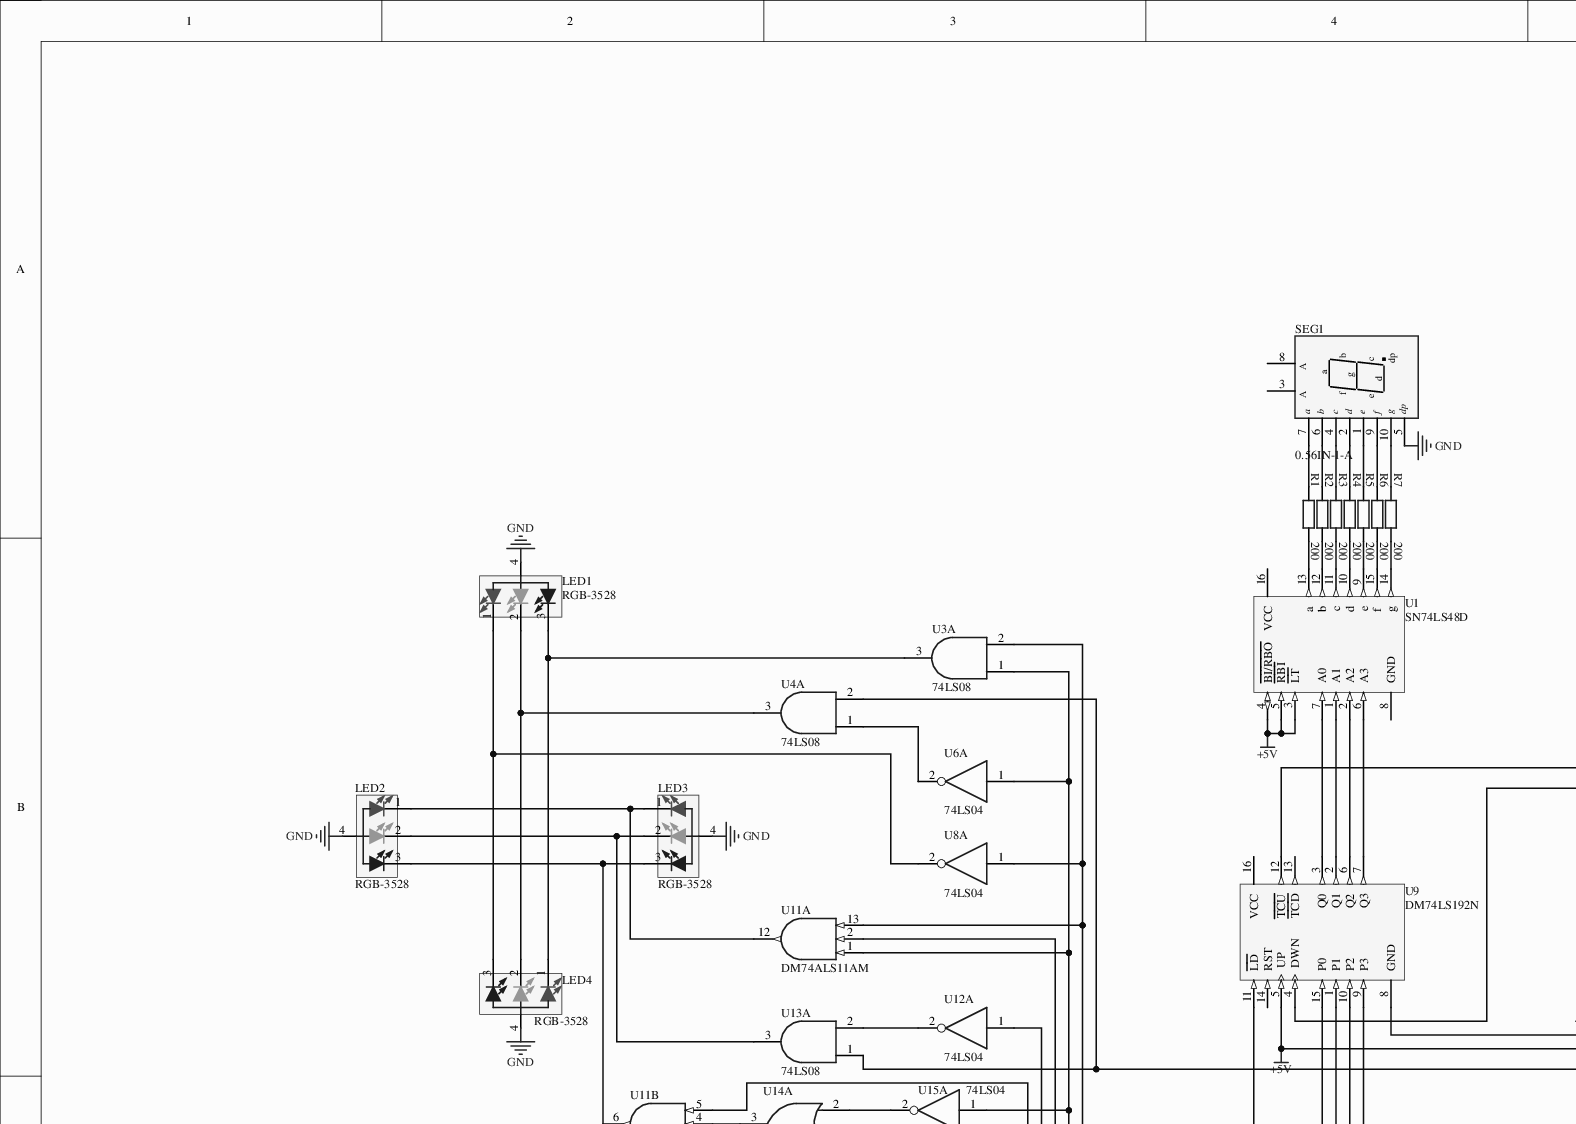
[diagram p0: MISC82158-6.SchDoc, top left]
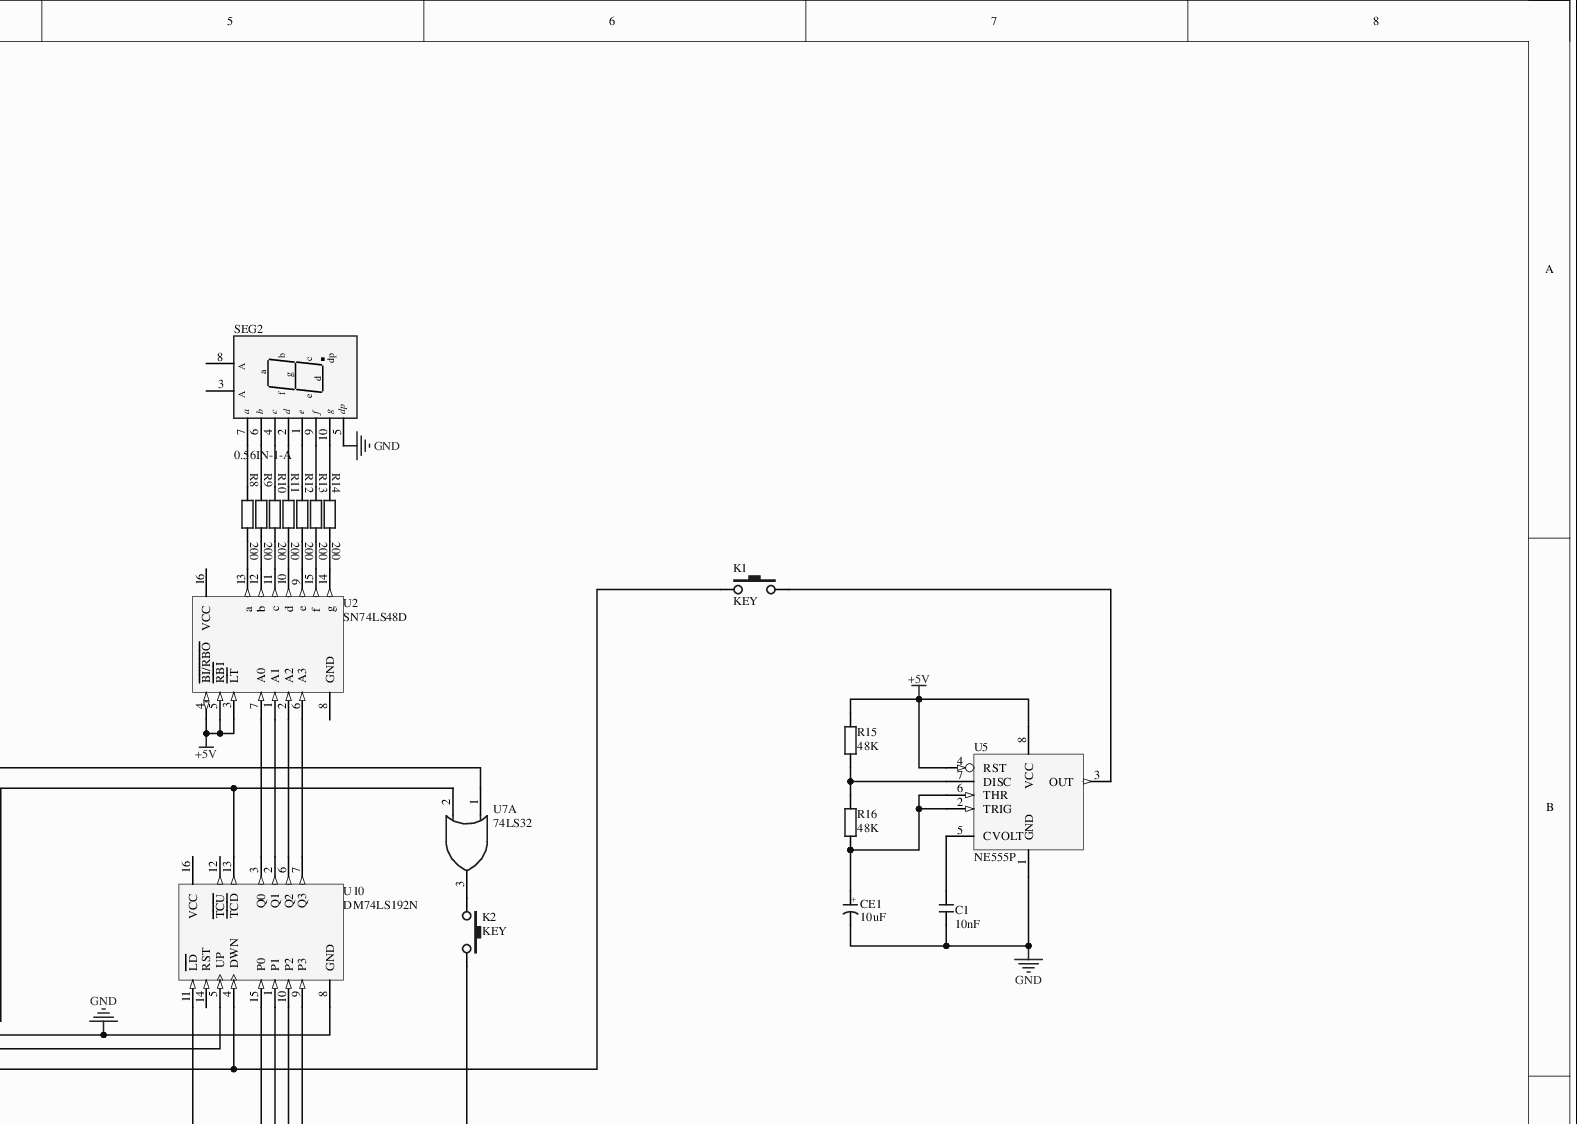
[diagram p1: MISC82158-6.SchDoc, top right]
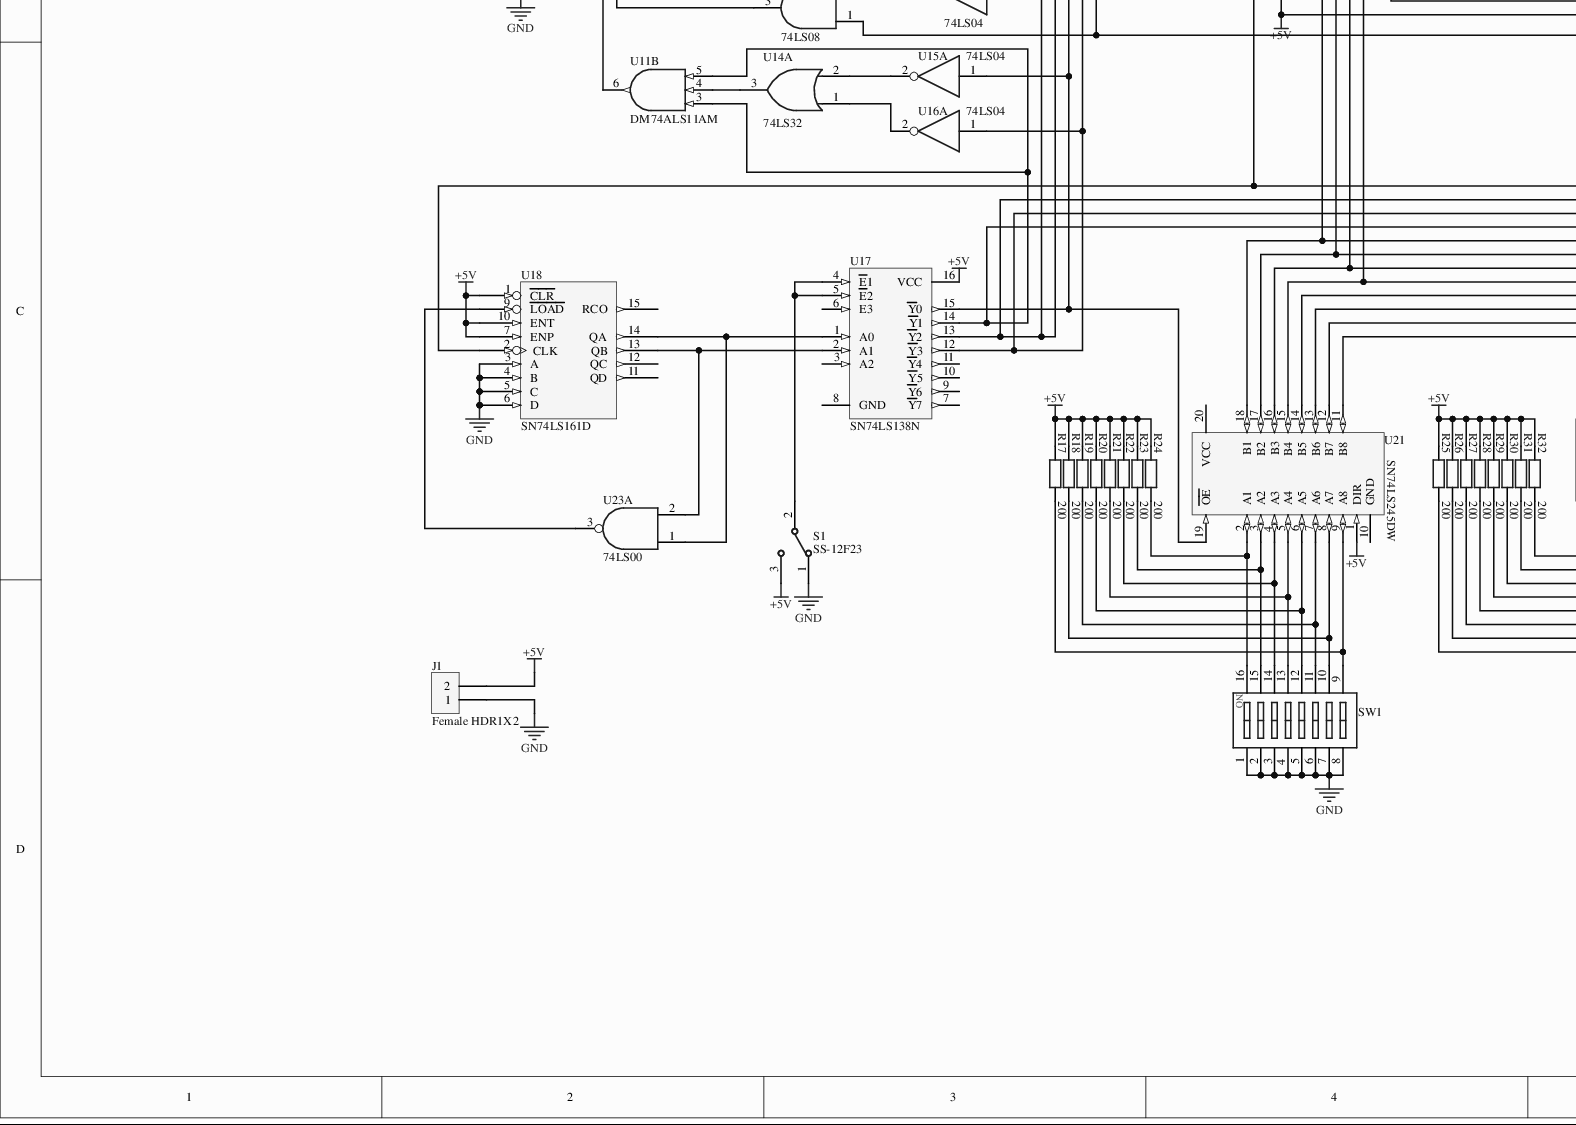
[diagram p2: MISC82158-6.SchDoc, bottom left]
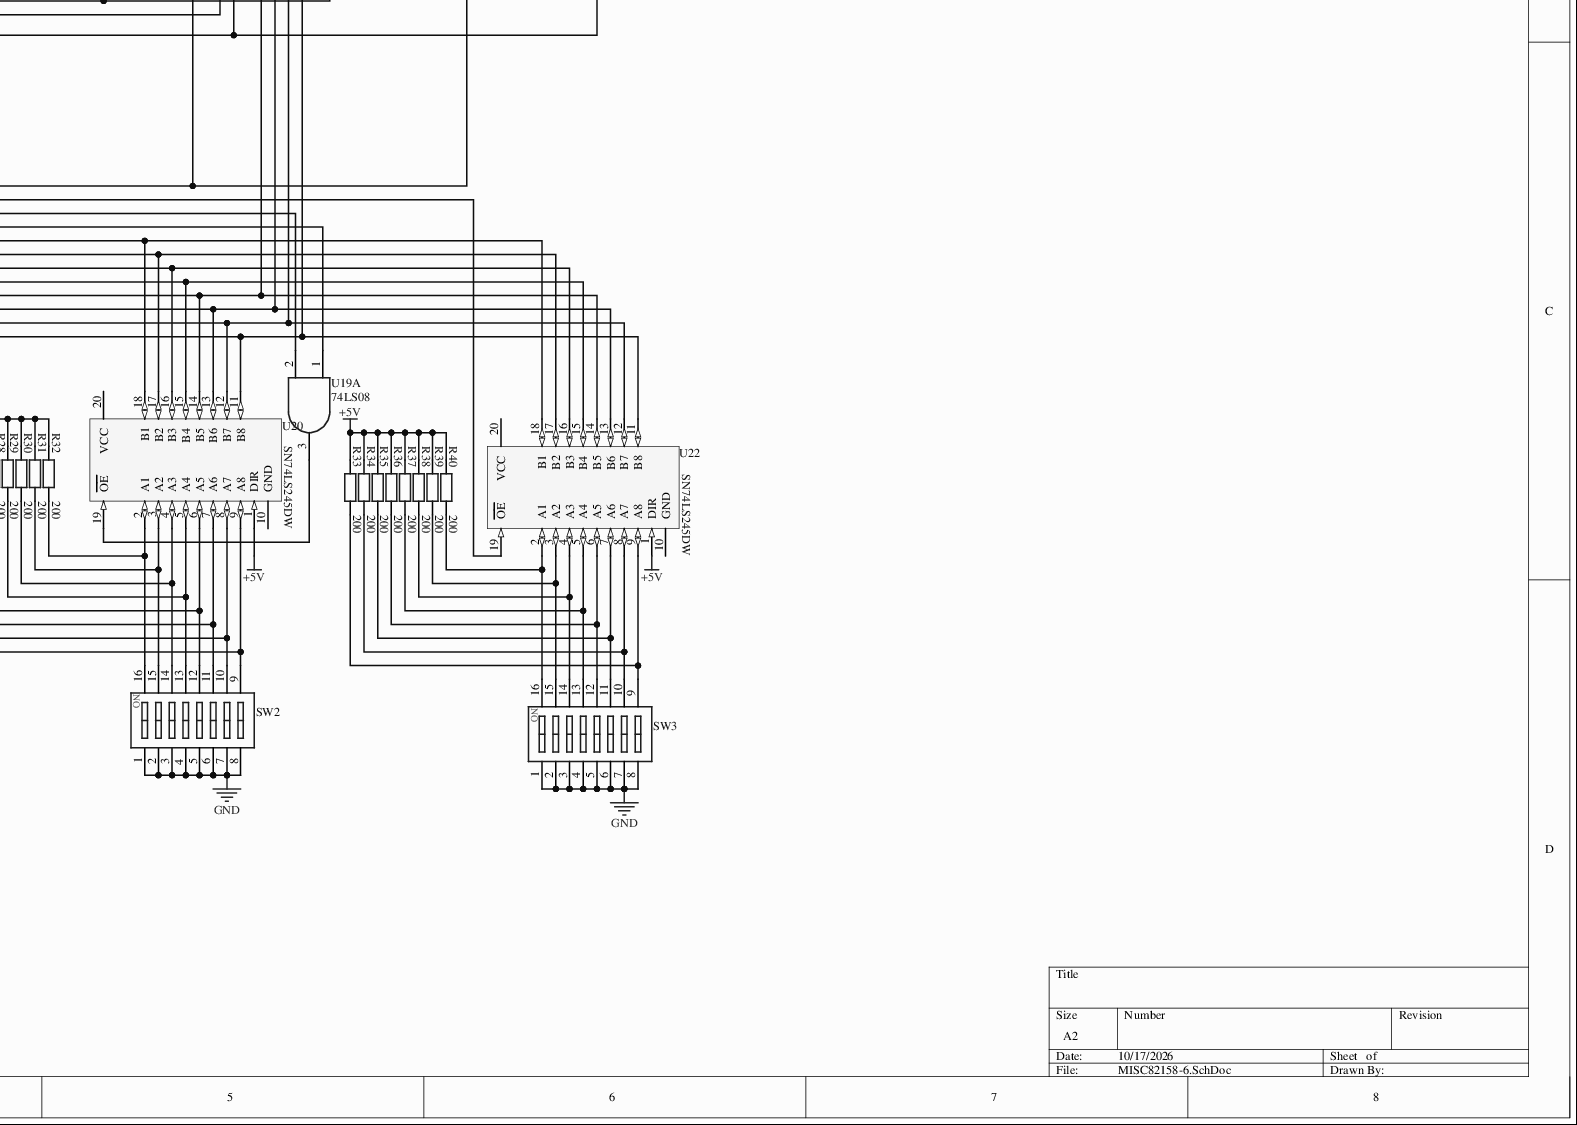
[diagram p3: MISC82158-6.SchDoc, bottom right]
# Altium project MISC82158-9.PrjPcb
1 sheet, 78 parts. Net scope: global (net labels, ports and power ports of the same name join across sheets).
Board file: MISC82158.PcbDoc

## Sheet MISC82158-6.SchDoc
size A2

### Parts
C1  10nF  [CC 1.8*3.6]
CE1  10uF  [CAP 1.5*4*8]
J1  Female HDR1X2  [Fe-HDR1X2/2.54-S]
K1  KEY  [DIP-3X6X4.3]
K2  KEY  [DIP-3X6X4.3]
LED1  RGB-3528  [Fe-HDR1X4/2.54-S]
LED2  RGB-3528  [Fe-HDR1X4/2.54-S]
LED3  RGB-3528  [Fe-HDR1X4/2.54-S]
LED4  RGB-3528  [Fe-HDR1X4/2.54-S]
R1  200  [RS 1/4W]
R2  200  [RS 1/4W]
R3  200  [RS 1/4W]
R4  200  [RS 1/4W]
R5  200  [RS 1/4W]
R6  200  [RS 1/4W]
R7  200  [RS 1/4W]
R8  200  [RS 1/4W]
R9  200  [RS 1/4W]
R10  200  [RS 1/4W]
R11  200  [RS 1/4W]
R12  200  [RS 1/4W]
R13  200  [RS 1/4W]
R14  200  [RS 1/4W]
R15  48K  [RS 1/4W]
R16  48K  [RS 1/4W]
R17  200  [RS 1/4W]
R18  200  [RS 1/4W]
R19  200  [RS 1/4W]
R20  200  [RS 1/4W]
R21  200  [RS 1/4W]
R22  200  [RS 1/4W]
R23  200  [RS 1/4W]
R24  200  [RS 1/4W]
R25  200  [RS 1/4W]
R26  200  [RS 1/4W]
R27  200  [RS 1/4W]
R28  200  [RS 1/4W]
R29  200  [RS 1/4W]
R30  200  [RS 1/4W]
R31  200  [RS 1/4W]
R32  200  [RS 1/4W]
R33  200  [RS 1/4W]
R34  200  [RS 1/4W]
R35  200  [RS 1/4W]
R36  200  [RS 1/4W]
R37  200  [RS 1/4W]
R38  200  [RS 1/4W]
R39  200  [RS 1/4W]
R40  200  [RS 1/4W]
S1  SS-12F23  [MSK-12C01-07]
SEG1  0.56IN-1-A  [0.56IN-1P]
SEG2  0.56IN-1-A  [0.56IN-1P]
SW1  SW-8P  [CSW DIP-8P]  (value not drawn)
SW2  SW-8P  [CSW DIP-8P]  (value not drawn)
SW3  SW-8P  [CSW DIP-8P]  (value not drawn)
U1  SN74LS48D  [SOP16]
U2  SN74LS48D  [SOP16]
U3  74LS08  [DIP14]  (part A of 4)
U4  74LS08  [DIP14]  (part A of 4)
U5  NE555P  [DIP8]
U6  74LS04  [DIP14]  (part A of 6)
U7  74LS32  [DIP14]  (part A of 4)
U8  74LS04  [DIP14]  (part A of 6)
U9  DM74LS192N  [DIP16]
U10  DM74LS192N  [DIP16]
U11  DM74ALS11AM  [DIP16]  (parts A,B of 3)
U12  74LS04  [DIP14]  (part A of 6)
U13  74LS08  [DIP14]  (part A of 4)
U14  74LS32  [DIP14]  (part A of 4)
U15  74LS04  [DIP14]  (part A of 6)
U16  74LS04  [DIP14]  (part A of 6)
U17  SN74LS138N  [DIP16]
U18  SN74LS161D  [DIP16]
U19  74LS08  [DIP14]  (part A of 4)
U20  SN74LS245DW  [SOP20]
U21  SN74LS245DW  [SOP20]
U22  SN74LS245DW  [SOP20]
U23  74LS00  [DIP14]  (part A of 4)

### Nets
+5V: J1.2 R15.1 R17.2 R18.2 R19.2 R20.2 R21.2 R22.2 R23.2 R24.2 R25.2 R26.2 R27.2 R28.2 R29.2 R30.2 R31.2 R32.2 R33.2 R34.2 R35.2 R36.2 R37.2 R38.2 R39.2 R40.2 S1.3 U1.3(~{LT}) U1.4(~{BI/RBO}) U1.5(~{RBI}) U2.3(~{LT}) U2.4(~{BI/RBO}) U2.5(~{RBI}) U5.4(RST) U5.8(VCC) U9.5(UP) U10.5(UP) U17.16(VCC) U18.1(~{CLR}) U18.7(ENP) U18.10(ENT) U20.1(DIR) U21.1(DIR) U22.1(DIR)
GND: C1.1 CE1.2(K) J1.1 LED1.4(A) LED2.4(A) LED3.4(A) LED4.4(A) S1.1 SEG1.5 SEG2.5 SW1.1 SW1.2 SW1.3 SW1.4 SW1.5 SW1.6 SW1.7 SW1.8 SW2.1 SW2.2 SW2.3 SW2.4 SW2.5 SW2.6 SW2.7 SW2.8 SW3.1 SW3.2 SW3.3 SW3.4 SW3.5 SW3.6 SW3.7 SW3.8 U5.1(GND) U9.8(GND) U10.8(GND) U11.7(GND) U18.3(A) U18.4(B) U18.5(C) U18.6(D) U18.8(GND)
VCC: U11.14(VCC) U18.16(VCC)
NetC1_2: C1.2 U5.5(CVOLT)
NetCE1_1: CE1.1(A) R16.2 U5.2(TRIG) U5.6(THR)
NetK1_1: K1.1 U4.2(B) U10.4(DWN) U13.1(A)
NetK1_3: K1.3 U5.3(OUT)
NetK2_1: K2.1 U7.3(Y)
NetK2_3: K2.3 U9.11(~{LD}) U10.11(~{LD}) U18.2(CLK)
NetLED1_1: LED1.1(RED_K) LED4.3(BULE_K) U8.2(Y)
NetLED1_2: LED1.2(GREEN_K) LED4.2(GREEN_K) U4.3(Y)
NetLED1_3: LED1.3(BULE_K) LED4.1(RED_K) U3.3(Y)
NetLED2_1: LED2.1(RED_K) LED3.1(RED_K) U11.12(Y)
NetLED2_2: LED2.2(GREEN_K) LED3.2(GREEN_K) U13.3(Y)
NetLED2_3: LED2.3(BULE_K) LED3.3(BULE_K) U11.6(Y)
NetR1_1: R1.1 U1.13(a)
NetR1_2: R1.2 SEG1.7
NetR2_1: R2.1 U1.12(b)
NetR2_2: R2.2 SEG1.6
NetR3_1: R3.1 U1.11(c)
NetR3_2: R3.2 SEG1.4
NetR4_1: R4.1 U1.10(d)
NetR4_2: R4.2 SEG1.2
NetR5_1: R5.1 U1.9(e)
NetR5_2: R5.2 SEG1.1
NetR6_1: R6.1 U1.15(f)
NetR6_2: R6.2 SEG1.9
NetR7_1: R7.1 U1.14(g)
NetR7_2: R7.2 SEG1.10
NetR8_1: R8.1 U2.13(a)
NetR8_2: R8.2 SEG2.7
NetR9_1: R9.1 U2.12(b)
NetR9_2: R9.2 SEG2.6
NetR10_1: R10.1 U2.11(c)
NetR10_2: R10.2 SEG2.4
NetR11_1: R11.1 U2.10(d)
NetR11_2: R11.2 SEG2.2
NetR12_1: R12.1 U2.9(e)
NetR12_2: R12.2 SEG2.1
NetR13_1: R13.1 U2.15(f)
NetR13_2: R13.2 SEG2.9
NetR14_1: R14.1 U2.14(g)
NetR14_2: R14.2 SEG2.10
NetR15_2: R15.2 R16.1 U5.7(DISC)
NetR17_1: R17.1 SW1.9 U21.9(A8)
NetR18_1: R18.1 SW1.10 U21.8(A7)
NetR19_1: R19.1 SW1.11 U21.7(A6)
NetR20_1: R20.1 SW1.12 U21.6(A5)
NetR21_1: R21.1 SW1.13 U21.5(A4)
NetR22_1: R22.1 SW1.14 U21.4(A3)
NetR23_1: R23.1 SW1.15 U21.3(A2)
NetR24_1: R24.1 SW1.16 U21.2(A1)
NetR25_1: R25.1 SW2.9 U20.9(A8)
NetR26_1: R26.1 SW2.10 U20.8(A7)
NetR27_1: R27.1 SW2.11 U20.7(A6)
NetR28_1: R28.1 SW2.12 U20.6(A5)
NetR29_1: R29.1 SW2.13 U20.5(A4)
NetR30_1: R30.1 SW2.14 U20.4(A3)
NetR31_1: R31.1 SW2.15 U20.3(A2)
NetR32_1: R32.1 SW2.16 U20.2(A1)
NetR33_1: R33.1 SW3.9 U22.9(A8)
NetR34_1: R34.1 SW3.10 U22.8(A7)
NetR35_1: R35.1 SW3.11 U22.7(A6)
NetR36_1: R36.1 SW3.12 U22.6(A5)
NetR37_1: R37.1 SW3.13 U22.5(A4)
NetR38_1: R38.1 SW3.14 U22.4(A3)
NetR39_1: R39.1 SW3.15 U22.3(A2)
NetR40_1: R40.1 SW3.16 U22.2(A1)
NetS1_2: S1.2 U17.4(~{E}1) U17.5(~{E}2)
NetU1_1: U1.1(A1) U9.2(Q1)
NetU1_2: U1.2(A2) U9.6(Q2)
NetU1_6: U1.6(A3) U9.7(Q3)
NetU1_7: U1.7(A0) U9.3(Q0)
NetU2_1: U2.1(A1) U10.2(Q1)
NetU2_2: U2.2(A2) U10.6(Q2)
NetU2_6: U2.6(A3) U10.7(Q3)
NetU2_7: U2.7(A0) U10.3(Q0)
NetU3_1: U3.1(A) U6.1(A) U11.1(A) U15.1(A) U17.15(~{Y}0) U21.19(~{OE})
NetU3_2: U3.2(B) U8.1(A) U11.13(C) U16.1(A) U17.12(~{Y}3) U19.2(B)
NetU4_1: U4.1(A) U6.2(Y)
NetU7_1: U7.1(A) U9.12(~{TCU})
NetU7_2: U7.2(B) U9.4(DWN) U10.13(~{TCD})
NetU9_1: U9.1(P1) U20.17(B2) U21.17(B2) U22.17(B2)
NetU9_9: U9.9(P3) U20.15(B4) U21.15(B4) U22.15(B4)
NetU9_10: U9.10(P2) U20.16(B3) U21.16(B3) U22.16(B3)
NetU9_15: U9.15(P0) U20.18(B1) U21.18(B1) U22.18(B1)
NetU10_1: U10.1(P1) U20.13(B6) U21.13(B6) U22.13(B6)
NetU10_9: U10.9(P3) U20.11(B8) U21.11(B8) U22.11(B8)
NetU10_10: U10.10(P2) U20.12(B7) U21.12(B7) U22.12(B7)
NetU10_15: U10.15(P0) U20.14(B5) U21.14(B5) U22.14(B5)
NetU11_2: U11.2(B) U12.1(A) U17.13(~{Y}2) U22.19(~{OE})
NetU11_3: U11.3(A) U11.5(C) U17.14(~{Y}1) U19.1(A)
NetU11_4: U11.4(B) U14.3(Y)
NetU12_2: U12.2(Y) U13.2(B)
NetU14_1: U14.1(A) U16.2(Y)
NetU14_2: U14.2(B) U15.2(Y)
NetU17_1: U17.1(A0) U18.14(QA) U23.1(A)
NetU17_2: U17.2(A1) U18.13(QB) U23.2(B)
NetU18_9: U18.9(~{LOAD}) U23.3(Y)
NetU19_3: U19.3(Y) U20.19(~{OE})

Not connected (* = marked no-connect by the designer): SEG1 3(VCC) 8; SEG2 3(VCC) 8; U1 8(GND) 16(VCC); U2 8(GND) 16(VCC); U3 7(GND) 14(VCC); U4 7(GND) 14(VCC); U6 7(GND) 14(VCC); U7 7(GND) 14(VCC); U8 7(GND) 14(VCC); U9 13(~{TCD}) 14(RST) 16(VCC); U10 12(~{TCU}) 14(RST) 16(VCC); U12 7(GND) 14(VCC); U13 7(GND) 14(VCC); U14 7(GND) 14(VCC); U15 7(GND) 14(VCC); U16 7(GND) 14(VCC); U17 3(A2)* 6(E3)* 7(~{Y}7) 8(GND) 9(~{Y}6) 10(~{Y}5) 11(~{Y}4); U18 11(QD) 12(QC) 15(RCO); U19 7(GND) 14(VCC); U20 10(GND) 20(VCC); U21 10(GND) 20(VCC); U22 10(GND) 20(VCC); U23 7(GND) 14(VCC)

### Library data of the parts
C1 = CC: Ceramic capacitor; BOM名称: Through-hole ceramic capacitor
CE1 = CE: Through-hole electrolytic capacitor; BOM名称: Through-hole electrolytic capacitor
LED1-LED4 = LED-RGB 3528: 3528 RGB LED; BOM名称: RGB LED
R1-R40 = R-S: Color-band resistor; BOM名称: Color-band resistor
S1 = SSW-1P: 1-way wave switch; BOM名称: Wave switch
SEG1 SEG2 = 0.56IN-1-A: 1-digit 0.56 inch common-anode display
SW1-SW3 = SW-8P: 8-way coded switch; BOM名称: 8-way coded switch
U1 U2 = SN74LS48D: BCD-to-Seven-Segment Decoder/Driver; Revision 1: 12-Jul-2000: SIM Model Added.; Revision 2: 17-Jul-2002: Re-released for DXP Platform.; Package Information: Latest Revision: Jan-1998; Published: 8-Jun-2000; Datasheet: 1988 TTL Logic Data Book (Mar-1988); Package Reference: D016; Publisher: Altium Limited
U3 U4 U13 U19 = 74LS08: Quad 2-input AND gate
U5 = NE555P: Precision Timer; Package Information: Latest Revision: Jun-1999; Code - JEDEC: MO-001-AN; Published: 16-Jan-2001; Revision: 17-Jul-2002: Re-released for DXP Platform.; Datasheet: Latest Revision: Feb-1992; Package Reference: P008; Publisher: Altium Limited
U6 U8 U12 U15 U16 = 74LS04: Hex inverter
U7 U14 = 74LS32: Quad 2-input OR gate
U9 U10 = DM74LS192N: Up/Down Decade Counter with Separate Up/Down Clock; Package Information: Latest Revision: 2000; Published: 15-Apr-2002; Datasheet: Latest Revision: Mar-1992; Package Reference: N16A; Publisher: Altium Limited
U11 = DM74ALS11AM: Triple 3-Input AND Gate; Package Information: Latest Revision: 2000; Published: 17-Jul-2002; Datasheet: Latest Revision: Feb-1998; Package Reference: M14A; Publisher: Altium Limited
U17 = SN74LS138N: 1-of-8 Decoder/Demultiplexer; Package Information: Latest Revision: Apr-2000; Code - JEDEC: MS-001-BB; Published: 15-Apr-2002; Datasheet: Latest Revision: Dec-1999; Package Reference: 648-08; Publisher: Altium Limited
U18 = SN74LS161A: SYN 4-BIT CNT
U20-U22 = SN74LS245DW: Octal Bus Transceiver; Published: 15-Apr-2002; Datasheet: Latest Revision: Dec-1999; Package Reference: 751D-05; Publisher: Altium Limited
U23 = 74LS00: Quad 2-input NAND gate